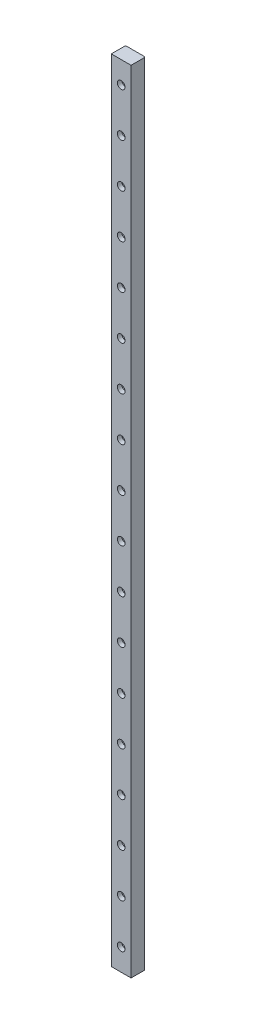
SolidWorks part; units mm, degrees
ref_plane "Front Plane" through (0, 0, 0) normal (0, 0, 1) x (1, 0, 0)
ref_plane "Top Plane" through (0, 0, 0) normal (0, 1, 0) x (1, 0, 0)
ref_plane "Right Plane" through (0, 0, 0) normal (1, 0, 0) x (0, 0, -1)
sketch "Sketch1" plane through (0, 0, 0) normal (0, 1, 0) x (1, 0, 0)
  line L1 (-4.5, 3.25) -> (4.5, 3.25)
  line L2 (-4.5, 3.25) -> (-4.5, -3.25)
  line L3 (-4.5, -3.25) -> (4.5, -3.25)
  line L4 (4.5, 3.25) -> (4.5, -3.25)
  line L5 (-4.5, 3.25) -> (4.5, -3.25) construction
  line L6 (-4.5, -3.25) -> (4.5, 3.25) construction
  point P0 (0, 0)
  dimension "D1" = 9
  dimension "D2" = 6.5
extrude "Boss-Extrude1" add sketch "Sketch1" along normal blind 360
chamfer "Chamfer1" distance 0.3 angle 45 2 edges at (-4.5, 180, -3.25) (4.5, 180, -3.25)
sketch "Sketch2" plane through (0, 0, -3.25) normal (0, 0, -1) x (-1, 0, 0)
  line L0 (0, 0) -> (0, 50000) construction
  line L1 (-4.2, 0) -> (4.2, 0) construction
  circle A0 centre (0, 10) radius 1.75
  dimension "D1" = 3.5
  dimension "D2" = 10
extrude "Cut-Extrude1" cut sketch "Sketch2" against normal blind 37
pattern_linear "LPattern1" count 18 spacing 20 along (0, 1, 0) of "Cut-Extrude1"
sketch "Sketch3" plane through (0, 0, -3.25) normal (0, 0, -1) x (-1, 0, 0)
  circle A0 centre (0, 10) radius 3
  dimension "D1" = 6
extrude "Cut-Extrude2" cut sketch "Sketch3" against normal blind 4.5
pattern_linear "LPattern2" count 18 spacing 20 along (0, 1, 0) of "Cut-Extrude2"
